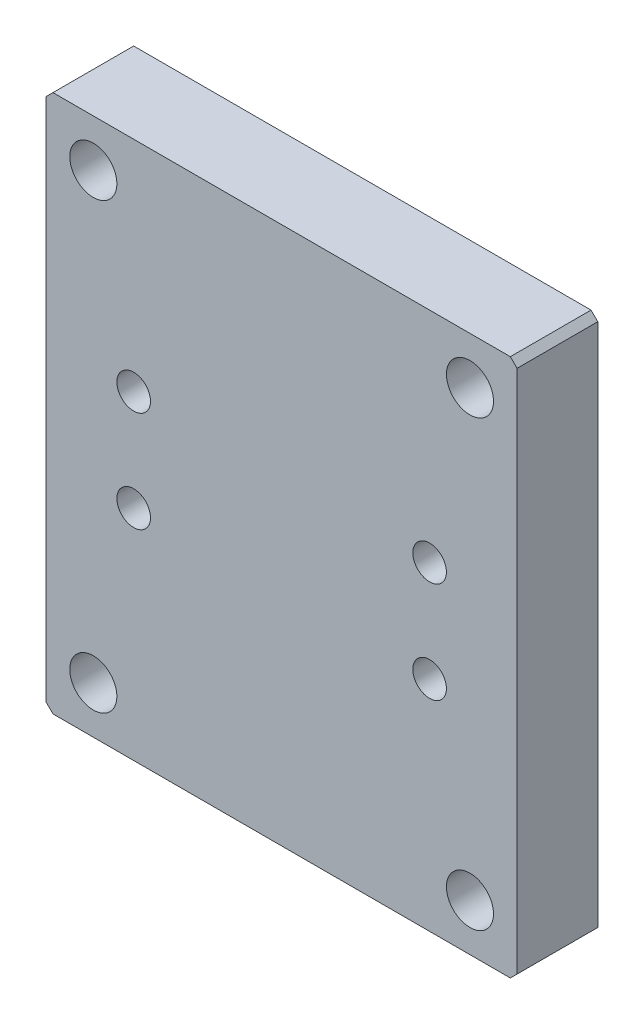
from build123d import *

# Parameters (mm, degrees)
SKETCH_1_W            = 70
SKETCH_1_H            = 80
EXTRUDE_1_DEPTH       = 12
CHAMFER_1_SIZE        = 1
HOLE_WIZARD_7_0_7_1_D = 7
HOLE_WIZARD_M6_1_D    = 5


with BuildPart() as part:
    # 草图1 → 凸台-拉伸1 (new body)
    with BuildSketch(Plane.XY):
        with Locations((35, -40)):
            Rectangle(SKETCH_1_W, SKETCH_1_H)
    extrude(amount=EXTRUDE_1_DEPTH)

    # 倒角1
    chamfer_1_edges = [part.edges().sort_by_distance(p)[0] for p in [
        (0, 0, 6),
        (70, 0, 6),
        (70, -80, 6),
        (0, -80, 6),
    ]]
    chamfer(chamfer_1_edges, length=CHAMFER_1_SIZE)

    # Ø7.0 (7) 直径孔1 (through all)
    with Locations(Plane(origin=(0, 0, 0), x_dir=(-1, 0, 0), z_dir=(0, 0, -1))):
        with Locations((-7, -73), (-7, -7), (-63, -73), (-63, -7)):
            Hole(HOLE_WIZARD_7_0_7_1_D / 2)

    # M6 螺纹孔1 (through all)
    with Locations(Plane(origin=(0, 0, 0), x_dir=(-1, 0, 0), z_dir=(0, 0, -1))):
        with Locations((-57, -32.5), (-57, -47.5), (-13, -47.5), (-13, -32.5)):
            Hole(HOLE_WIZARD_M6_1_D / 2)


solid = part.part
